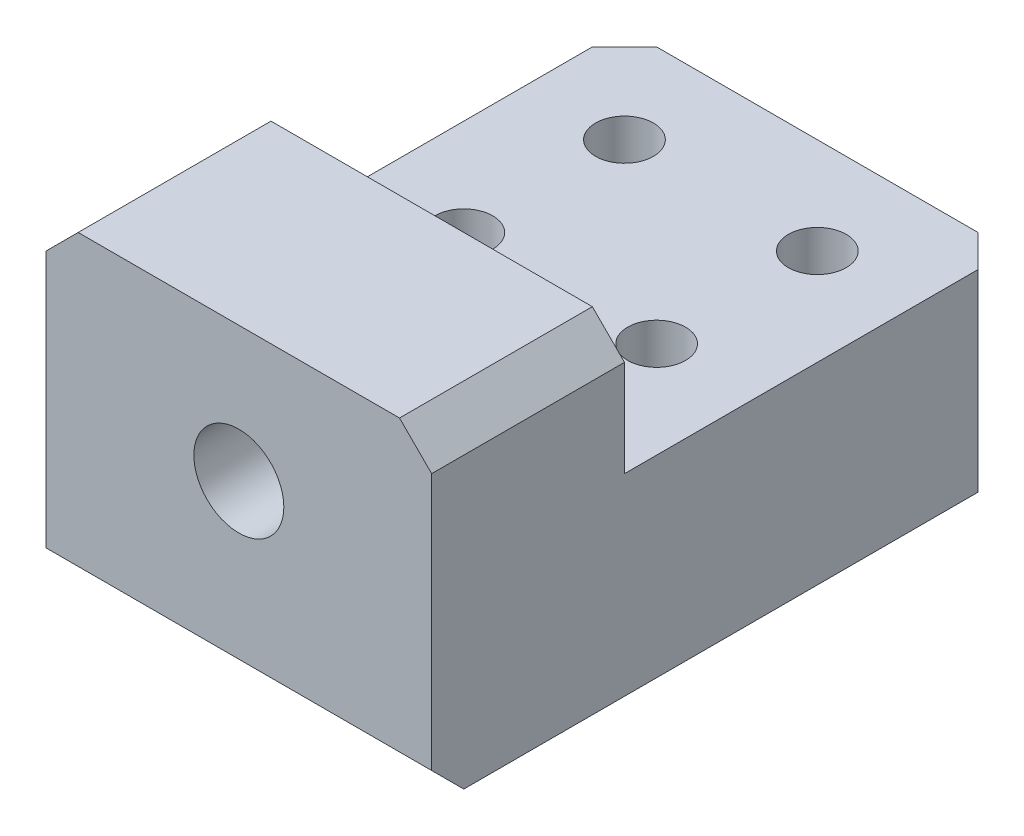
from build123d import *

# Parameters (mm, degrees)
SKETCH_1_W              = 60
SKETCH_1_H              = 30
EXTRUDE_1_DEPTH         = 90
SKETCH_2_W              = 60
SKETCH_2_H              = 30
EXTRUDE_2_DEPTH         = 20
HOLE_WIZARD_9_0_9_1_D   = 9
HOLE_WIZARD_M16_1_D     = 14
HOLE_WIZARD_M16_1_DEPTH = 38
HOLE_WIZARD_M16_1_TIP   = 4.206024333
CHAMFER_1_SIZE          = 5
CHAMFER_2_SIZE          = 5


with BuildPart() as part:
    # 草图1 → 凸台-拉伸1 (new body)
    with BuildSketch(Plane.XY):
        Rectangle(SKETCH_1_W, SKETCH_1_H)
    extrude(amount=EXTRUDE_1_DEPTH)

    # 草图2 → 凸台-拉伸2 (add)
    with BuildSketch(Plane(origin=(0, 15, 0), x_dir=(1, 0, 0), z_dir=(0, 1, 0))):
        with Locations((0, -75)):
            Rectangle(SKETCH_2_W, SKETCH_2_H)
    extrude(amount=EXTRUDE_2_DEPTH)

    # Ø9.0 (9) 直径孔1 (through all)
    with Locations(Plane(origin=(0, 15, 0), x_dir=(1, 0, 0), z_dir=(0, 1, 0))):
        with Locations((-15, -15), (15, -15), (-15, -40), (15, -40)):
            Hole(HOLE_WIZARD_9_0_9_1_D / 2)

    # M16 螺纹孔1
    with Locations(Plane.XY.offset(90)):
        with Locations((0, 14)):
            Hole(HOLE_WIZARD_M16_1_D / 2, depth=HOLE_WIZARD_M16_1_DEPTH)
            with Locations((0, 0, -(HOLE_WIZARD_M16_1_DEPTH + HOLE_WIZARD_M16_1_TIP / 2))):  # 118° drill point
                Cone(0, HOLE_WIZARD_M16_1_D / 2, HOLE_WIZARD_M16_1_TIP, mode=Mode.SUBTRACT)

    # 倒角1
    chamfer_1_edges = [part.edges().sort_by_distance(p)[0] for p in [
        (-30, 35, 75),
        (30, 35, 75),
        (-30, 0, 0),
        (30, 0, 0),
    ]]
    chamfer(chamfer_1_edges, length=CHAMFER_1_SIZE)

    # 倒角2
    chamfer_2_edges = [part.edges().sort_by_distance(p)[0] for p in [
        (0, -15, 90),
    ]]
    chamfer(chamfer_2_edges, length=CHAMFER_2_SIZE)


solid = part.part
